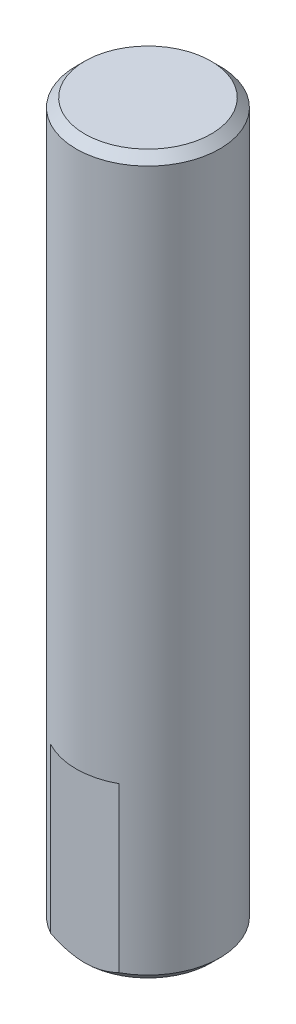
from build123d import *

# Parameters (mm, degrees)
SKETCH1_R           = 2.5
BOSS_EXTRUDE1_DEPTH = 25
CHAMFER1_SIZE       = 0.3
SKETCH3_W           = 4.032252552
SKETCH3_H           = 0.6
CUT_EXTRUDE2_DEPTH  = 6


with BuildPart() as part:
    # Sketch1 → Boss-Extrude1 (new body)
    with BuildSketch(Plane(origin=(0, 0, 0), x_dir=(1, 0, 0), z_dir=(0, 1, 0))):
        with Locations(Location((0, 0, 0), (0, 0, 270))):
            Circle(SKETCH1_R)
    extrude(amount=BOSS_EXTRUDE1_DEPTH)

    # Chamfer1
    chamfer1_edges = [part.edges().sort_by_distance(p)[0] for p in [
        (0, 0, -2.5),
        (0, 25, -2.5),
    ]]
    chamfer(chamfer1_edges, length=CHAMFER1_SIZE)

    # Sketch3 → Cut-Extrude2 (cut)
    with BuildSketch(Plane.XZ):
        with Locations((0, 2.5)):
            Rectangle(SKETCH3_W, SKETCH3_H)
    extrude(amount=-CUT_EXTRUDE2_DEPTH, mode=Mode.SUBTRACT)


solid = part.part
